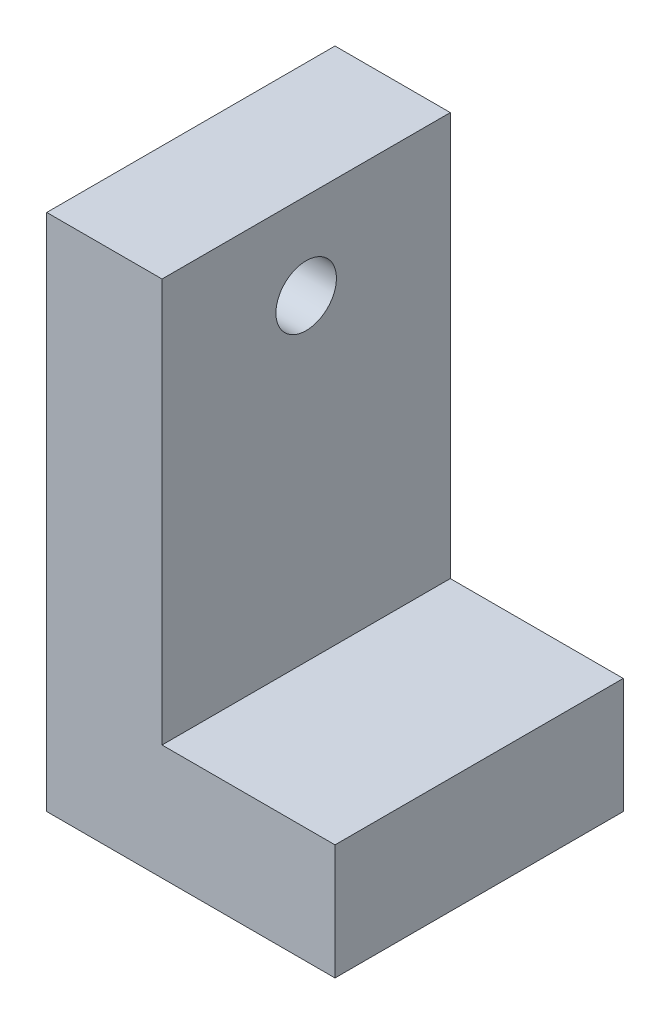
from build123d import *

# Parameters (mm, degrees)
EXTRUDE_1_DEPTH    = 10
HOLE_WIZARD_M5_1_D = 4.2


with BuildPart() as part:
    # 草图1 → 凸台-拉伸1 (new, symmetric)
    with BuildSketch(Plane.XY):
        Polygon((0, 0), (-20, 0), (-20, 36), (-12, 36), (-12, 8), (0, 8), align=None)
    extrude(amount=EXTRUDE_1_DEPTH, both=True)

    # M5 螺纹孔1 (through all)
    with Locations(Plane(origin=(-20, 30, 0), x_dir=(0, 0, -1), z_dir=(-1, 0, 0))):
        with Locations((0, 0)):
            Hole(HOLE_WIZARD_M5_1_D / 2)


solid = part.part
